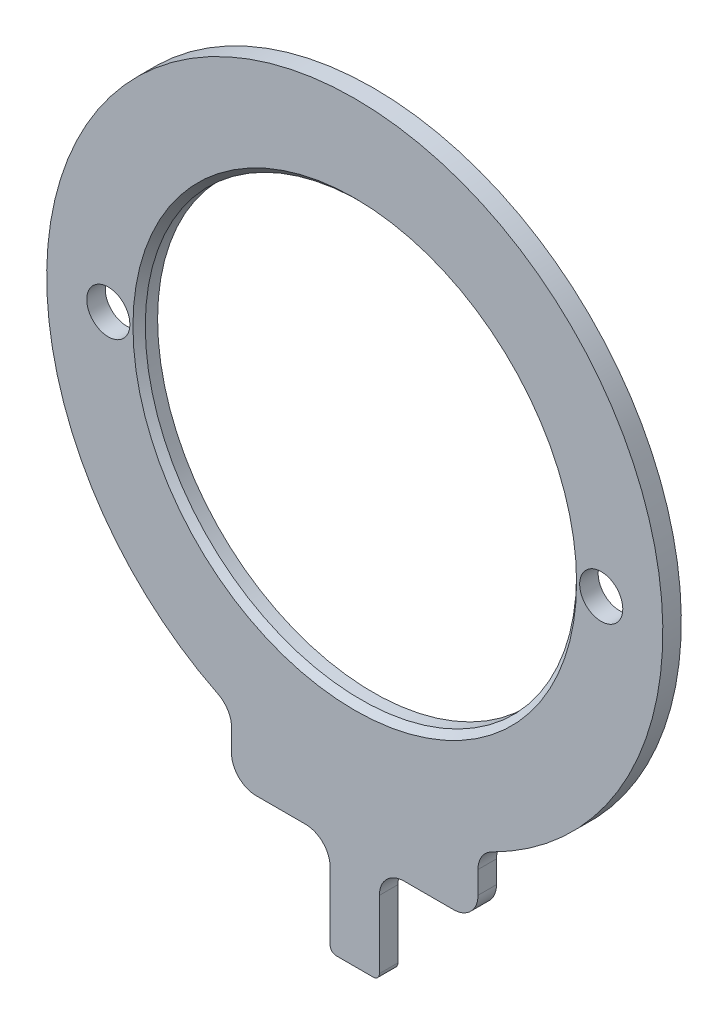
from build123d import *

# Parameters (mm, degrees)
SKETCH_1_R          = 25
SKETCH_1_R_2        = 17.5
EXTRUDE_1_DEPTH     = 1.5
SKETCH_4_W          = 20
SKETCH_4_H          = 15
EXTRUDE_2_DEPTH     = 1.5
SKETCH_5_W          = 8
SKETCH_5_H          = 8
CUT_EXTRUDE_3_DEPTH = 20
FILLET_2_R          = 2
SKETCH_6_R          = 1.75
CUT_EXTRUDE_4_DEPTH = 40
FILLET_3_R          = 0.5
CHAMFER_1_SIZE      = 0.5


with BuildPart() as part:
    # 草图1 → 凸台-拉伸1 (new body)
    with BuildSketch(Plane.XY):
        Circle(SKETCH_1_R)
        Circle(SKETCH_1_R_2, mode=Mode.SUBTRACT)
    extrude(amount=EXTRUDE_1_DEPTH)

    # 草图4 → 凸台-拉伸2 (add)
    with BuildSketch(Plane.XY.offset(1.5)):
        with Locations((0, -28.5)):
            Rectangle(SKETCH_4_W, SKETCH_4_H)
    extrude(amount=-EXTRUDE_2_DEPTH)

    # 草图5 → 切除-拉伸3 (cut)
    with BuildSketch(Plane.XY.offset(1.5)):
        with Locations((-6, -32)):
            Rectangle(SKETCH_5_W, SKETCH_5_H)
        with Locations((6, -32)):
            Rectangle(SKETCH_5_W, SKETCH_5_H)
    extrude(amount=-CUT_EXTRUDE_3_DEPTH, mode=Mode.SUBTRACT)

    # 圆角2
    fillet_2_edges = [part.edges().sort_by_distance(p)[0] for p in [
        (10, -22.912878475, 0.75),
        (-10, -22.912878475, 0.75),
        (-10, -28, 0.75),
        (-2, -28, 0.75),
        (2, -28, 0.75),
        (10, -28, 0.75),
    ]]
    fillet(fillet_2_edges, radius=FILLET_2_R)

    # 草图6 → 切除-拉伸4 (cut)
    with BuildSketch(Plane.XY.offset(1.5)):
        with Locations((-20, 0)):
            Circle(SKETCH_6_R)
        with Locations((20, 0)):
            Circle(SKETCH_6_R)
    extrude(amount=-CUT_EXTRUDE_4_DEPTH, mode=Mode.SUBTRACT)

    # 圆角3
    fillet_3_edges = [part.edges().sort_by_distance(p)[0] for p in [
        (-2, -36, 0.75),
        (2, -36, 0.75),
    ]]
    fillet(fillet_3_edges, radius=FILLET_3_R)

    # 倒角1
    chamfer_1_edges = [part.edges().sort_by_distance(p)[0] for p in [
        (-17.5, 0, 1.5),
    ]]
    chamfer(chamfer_1_edges, length=CHAMFER_1_SIZE)


solid = part.part
